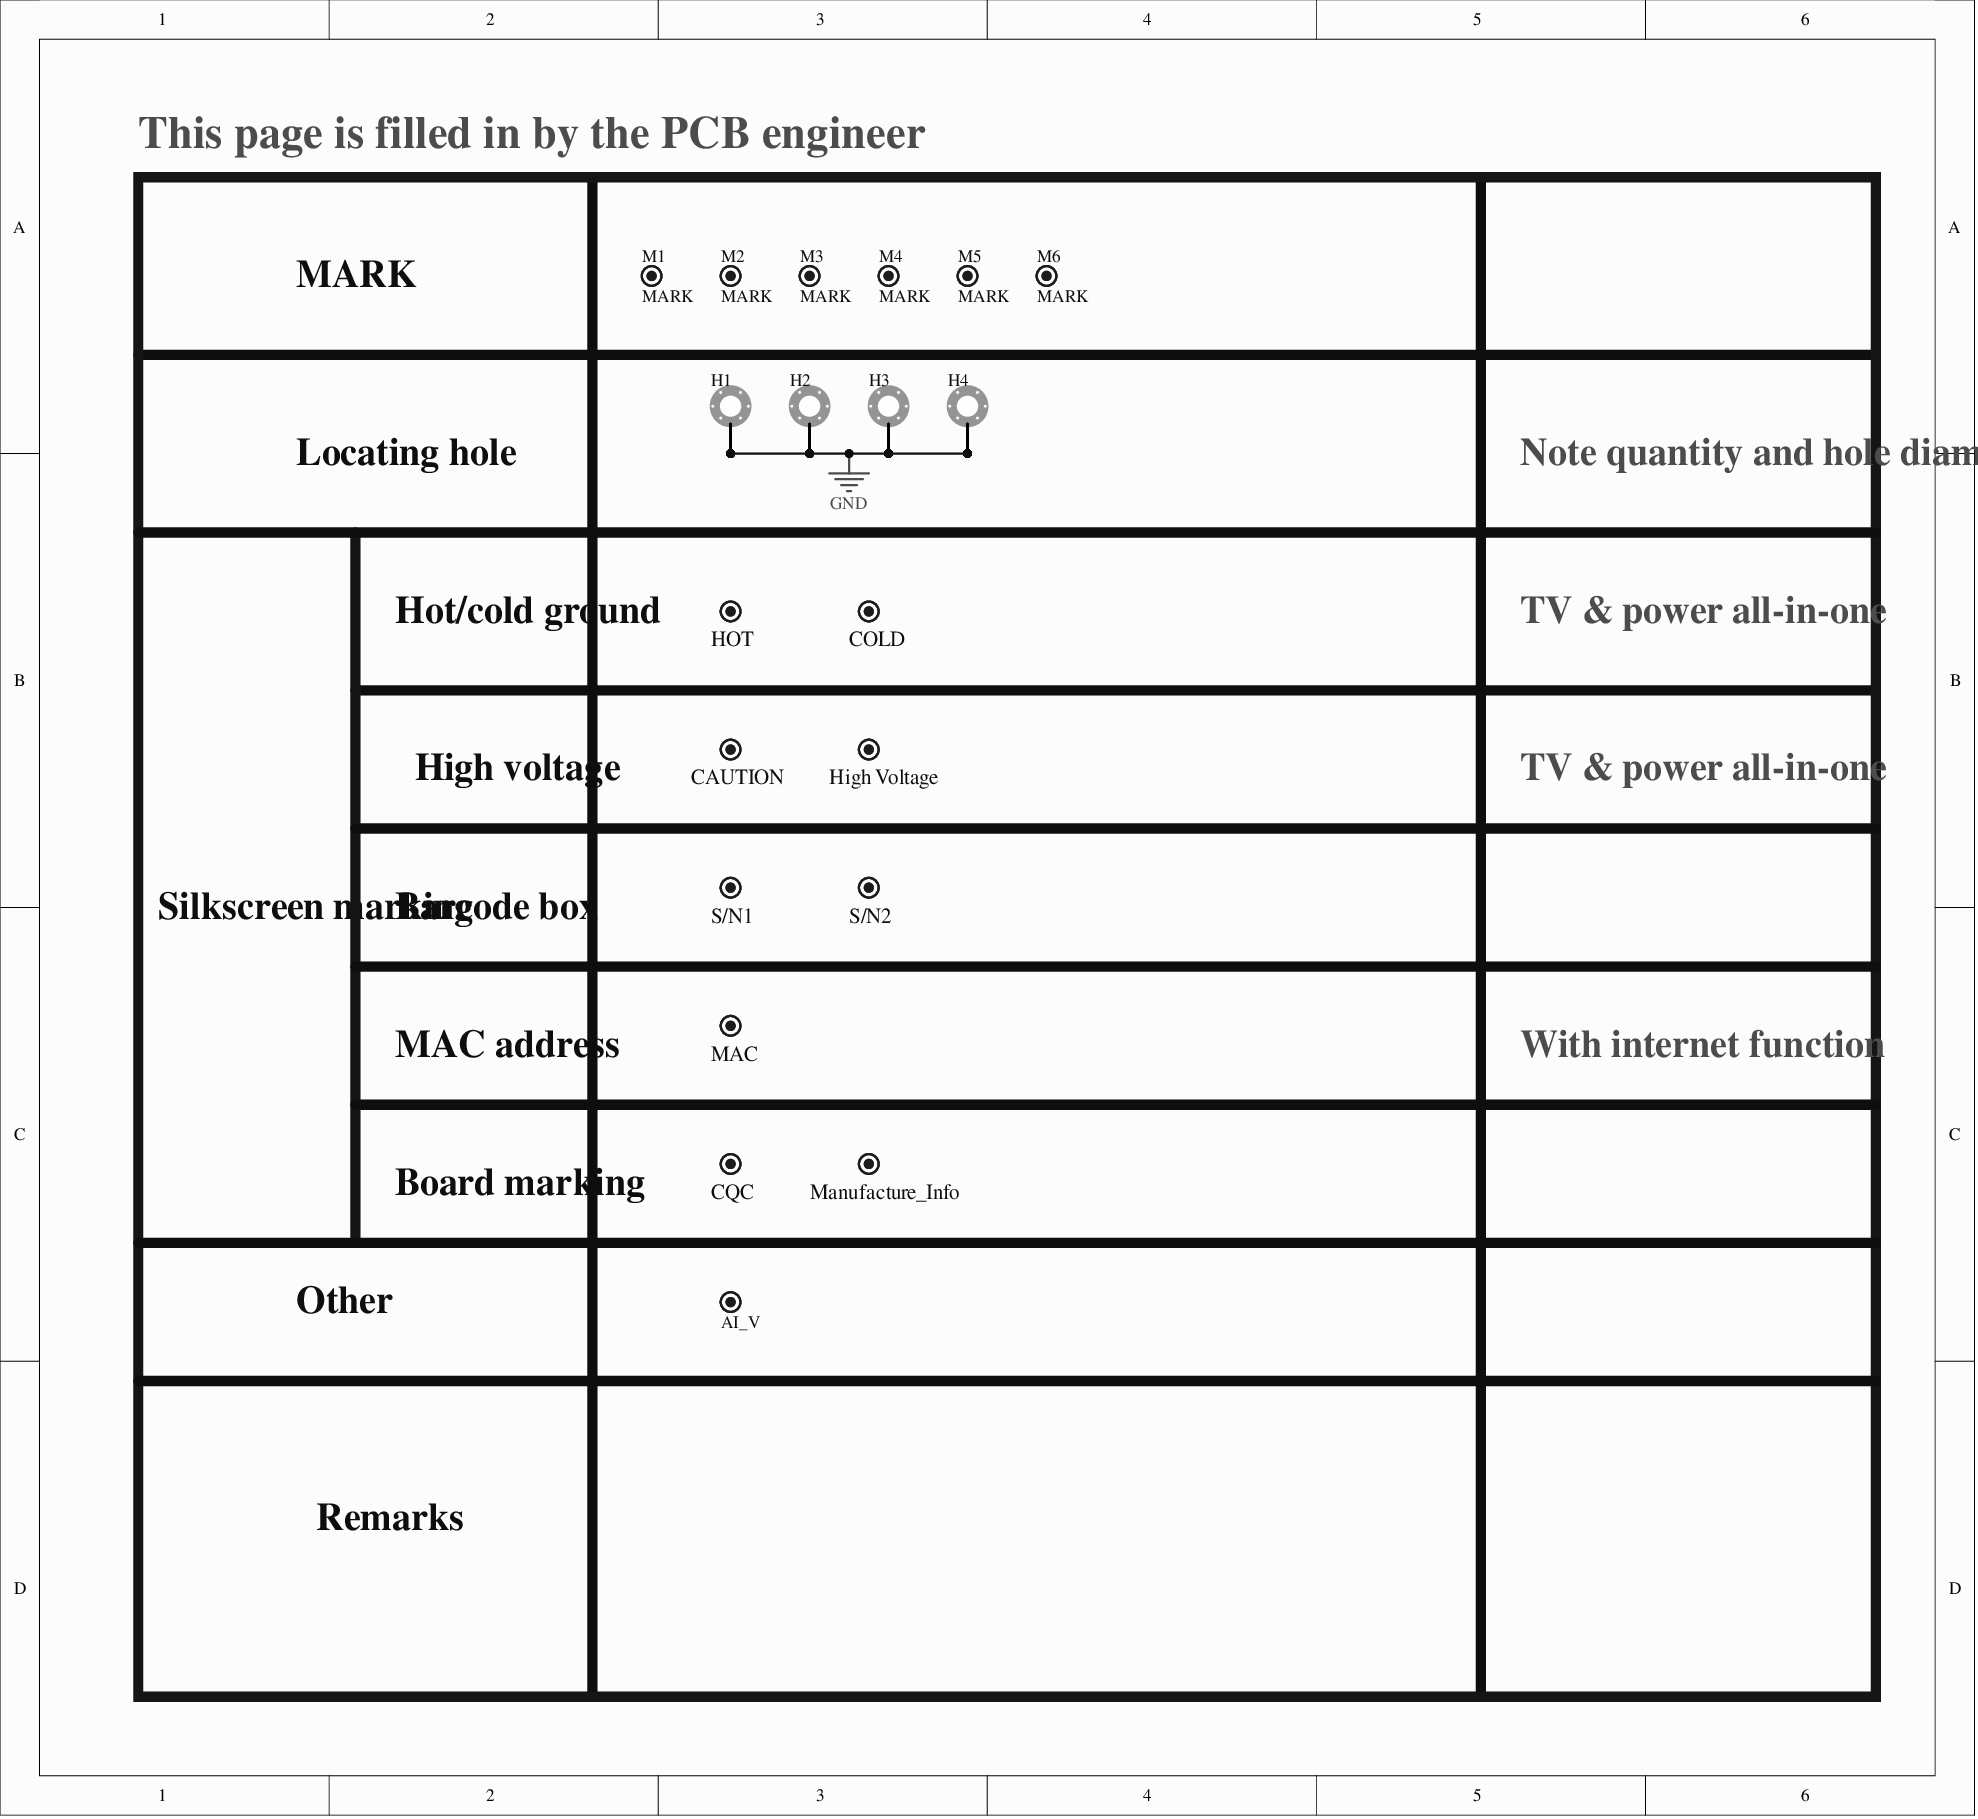
[diagram p0: MISC84395-3.SchDoc]
# Altium project MISC84395-37.PrjPCB (part 1 of 13)
17 sheets, 951 parts. Net scope: global (net labels, ports and power ports of the same name join across sheets).
Board file: MISC84395.PcbDoc
Sheets:
  MISC84395-3.SchDoc
  MISC84395-5.SchDoc
  MISC84395-2.schdoc
  MISC84395-7.SchDoc
  MISC84395-8.SchDoc
  MISC84395-9.SchDoc
  MISC84395-10.SchDoc
  MISC84395-11.SchDoc
  MISC84395-12.SchDoc
  MISC84395-13.SchDoc
  MISC84395-14.SchDoc
  MISC84395-15.SchDoc
  MISC84395-16.SchDoc
  MISC84395-17.SchDoc
  MISC84395-18.SchDoc
  MISC84395-4.SchDoc
  MISC84395-19.SchDoc

## Sheet MISC84395-3.SchDoc
size 254 x 233 mm

### Parts
AI_V  AI_GRIPPER_V  [AI_GRIPPER_V]  (value not drawn)
CAUTION  CAUTION  [CAUTION]
COLD  COLD  [COLD]
CQC  CQC  [CQC]
H1  Location hole  [ASSE4.0C-3]  (value not drawn)
H2  Location hole  [ASSE4.0C-3]  (value not drawn)
H3  Location hole  [ASSE4.0C-3]  (value not drawn)
H4  Location hole  [ASSE4.0C-3]  (value not drawn)
High_Voltage  High Voltage  [High Voltage]
HOT  HOT  [HOT]
M1  MARK  [MARK]
M2  MARK  [MARK]
M3  MARK  [MARK]
M4  MARK  [MARK]
M5  MARK  [MARK]
M6  MARK  [MARK]
MAC  MAC  [Barcode]  (value not drawn)
Manufacture_Info  Manufacture_Info  [Manufacture_Info]
S/N1  Barcode  [Barcode]  (value not drawn)
S/N2  Barcode  [Barcode]  (value not drawn)

### Nets
GND: H1.1 H1.2 H1.3 H1.4 H1.5 H1.6 H2.1 H2.2 H2.3 H2.4 H2.5 H2.6 H3.1 H3.2 H3.3 H3.4 H3.5 H3.6 H4.1 H4.2 H4.3 H4.4 H4.5 H4.6

### Notes on the sheet
- This page is filled in by the PCB engineer
- MARK
- Locating hole
- Note quantity and hole diameter
- (near HOT) Hot/cold ground
- TV & power all-in-one
- High voltage
- Silkscreen marking
- Barcode box
- MAC address
- With internet function
- Board marking
- Other
- Remarks

### Library data of the parts
H1-H4 = Location hole-D
M1-M6 = MARK-D
MAC = Barcode

## Sheet MISC84395-5.SchDoc
size 254 x 322 mm
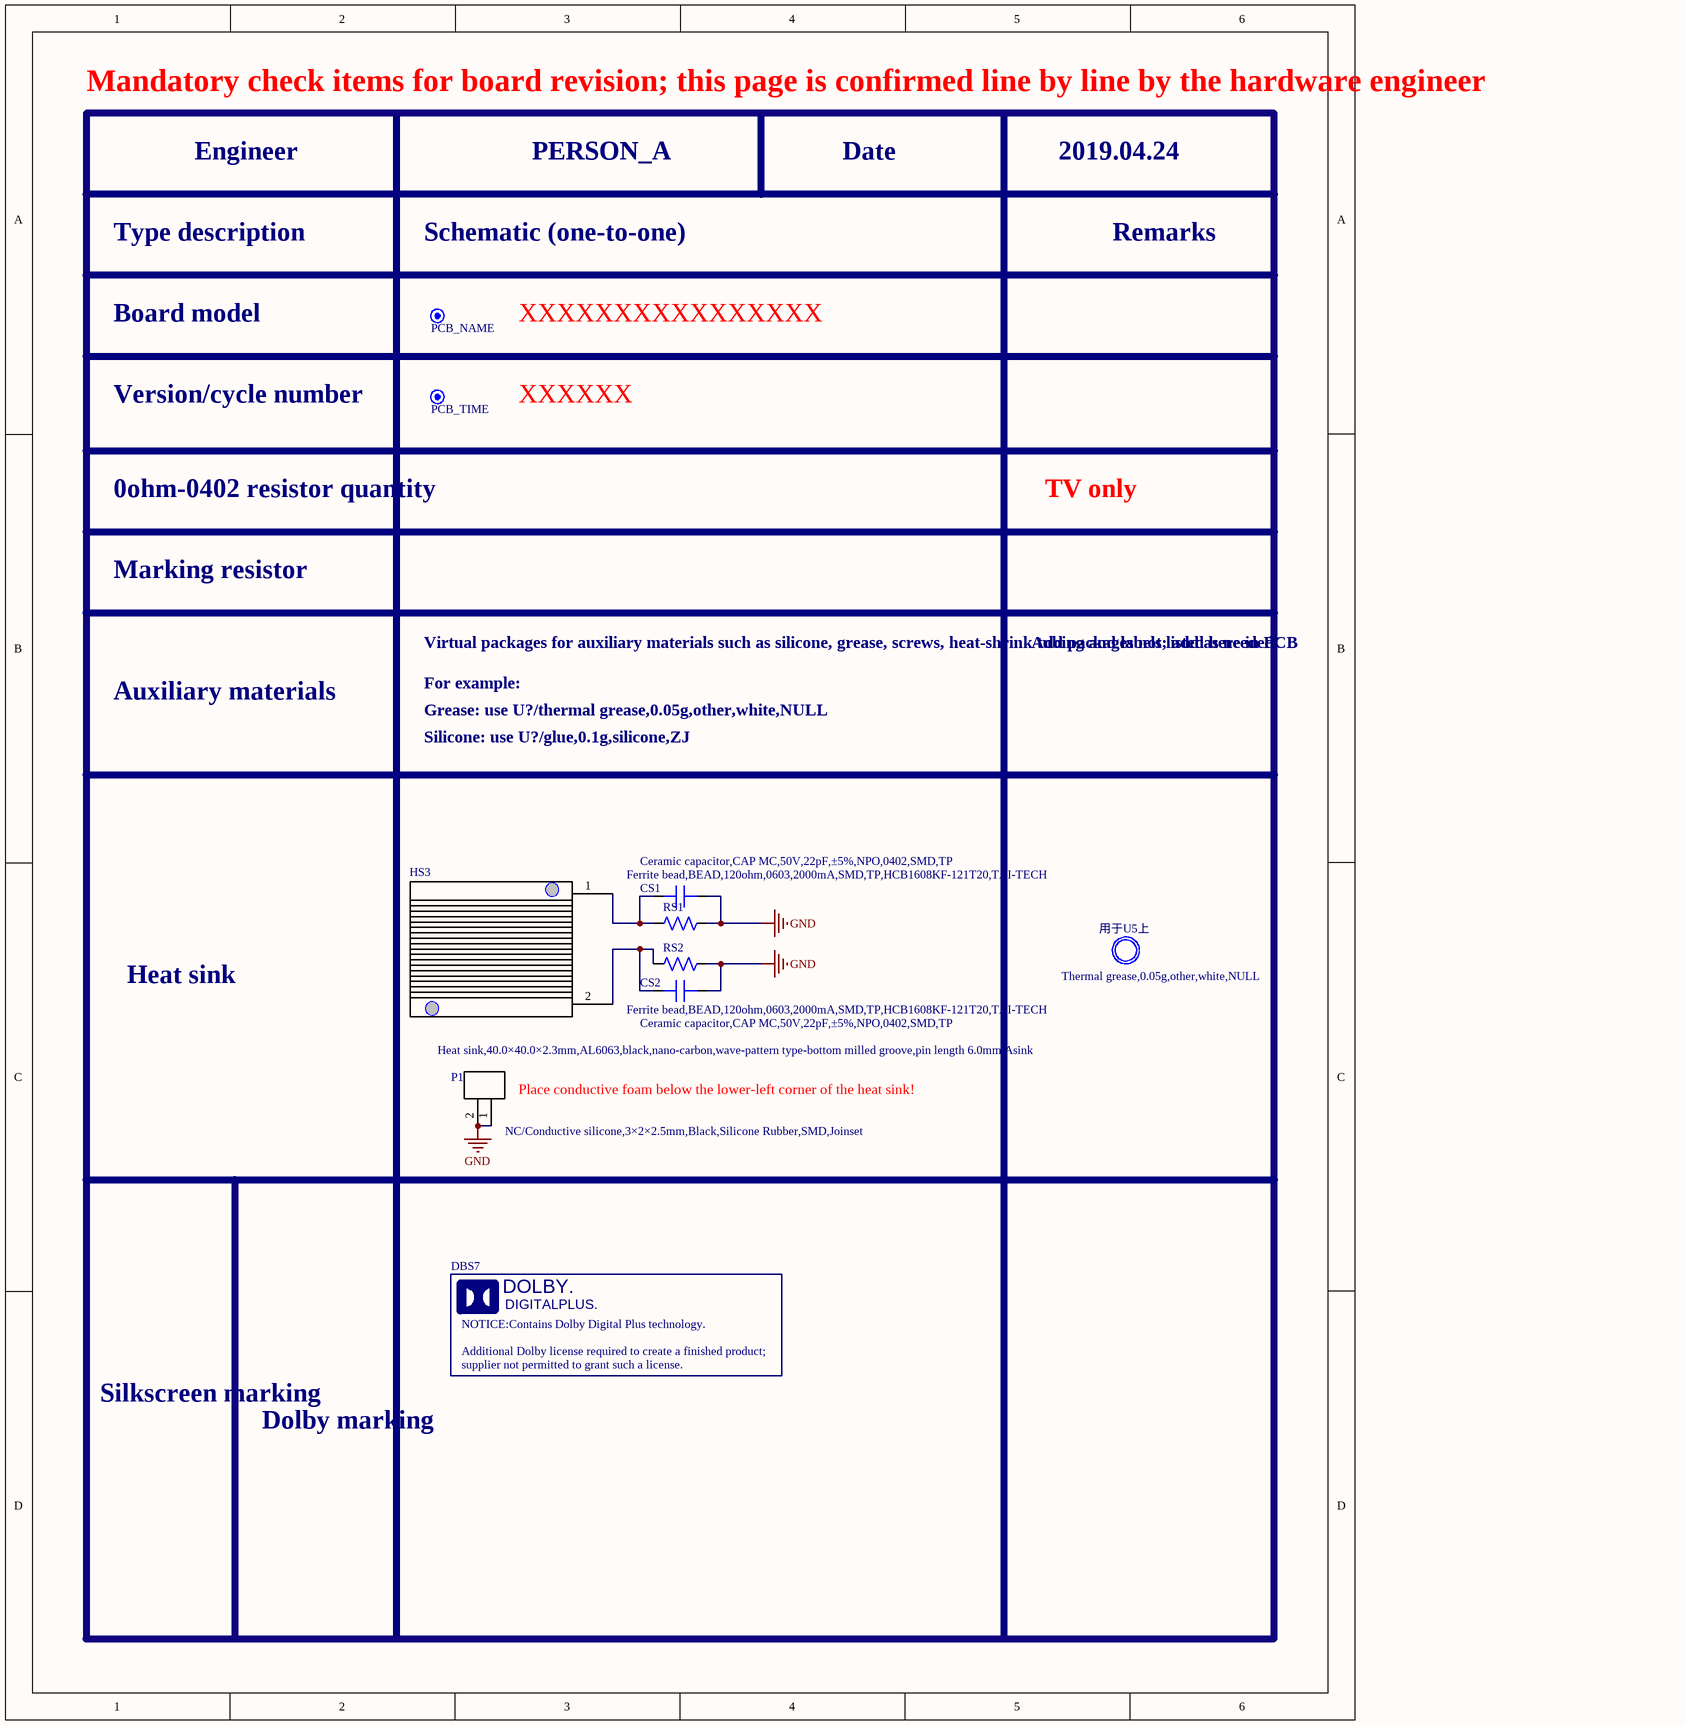
[diagram p1: MISC84395-5.SchDoc]

### Parts
CS1  Ceramic capacitor,CAP MC,50V,22pF,±5%,NPO,0402,SMD,TP  [C0402]
CS2  Ceramic capacitor,CAP MC,50V,22pF,±5%,NPO,0402,SMD,TP  [C0402]
DBS7  DOLBY PLUS  [DOLBY PLUS-SILK]  (value not drawn)
HS3  Heat sink,40.0×40.0×2.3mm,AL6063,black,nano-carbon,wave-pattern type-bottom milled groove,pin length 6.0mm,Asink  [HS(40*40*2.3)-1]
P1  NC/Conductive silicone,3×2×2.5mm,Black,Silicone Rubber,SMD,Joinset  [Silica gel(3*2*2.5)]
RS1  Ferrite bead,BEAD,120ohm,0603,2000mA,SMD,TP,HCB1608KF-121T20,TAI-TECH  [R0603]
RS2  Ferrite bead,BEAD,120ohm,0603,2000mA,SMD,TP,HCB1608KF-121T20,TAI-TECH  [R0603]
XXXXXX  PCB_TIME  [PCB_TIME]
XXXXXXXXXXXXXXXX  PCB_NAME  [PCB_NAME]
用于U5上  Thermal grease,0.05g,other,white,NULL  [Heat-Shrinkable Tube]

### Nets
GND: CS1.2 CS2.2 P1.1 P1.2 RS1.1 RS2.2
NetCS1_1: CS1.1 HS3.1 RS1.2
NetCS2_1: CS2.1 HS3.2 RS2.1

### Notes on the sheet
- Mandatory check items for board revision; this page is confirmed line by line by the hardware engineer
- Engineer
- PERSON_A
- Date
- 2019.04.24
- Type description
- Schematic (one-to-one)
- Remarks
- Board model
- Version/cycle number
- 0ohm-0402 resistor quantity
- TV only
- Marking resistor
- Virtual packages for auxiliary materials such as silicone, grease, screws, heat-shrink tubing and labels; add as needed
- Add packages not listed here in PCB
- Auxiliary materials
- For example:
- Grease: use U?/thermal grease,0.05g,other,white,NULL
- Silicone: use U?/glue,0.1g,silicone,ZJ
- Heat sink
- (near P1) Place conductive foam below the lower-left corner of the heat sink!
- Silkscreen marking
- Dolby marking

### Library data of the parts
CS1 CS2 = 1000pF-0402-X7R-±10%-50V-D
HS3 = 004.040.0002110-DLMI: Heat sink,AL6063,40.0×40.0×2.3mm,black,nano-carbon,wave-pattern type-bottom milled groove,Asink-DLMI
P1 = 导电硅胶,3×2×2.5mm,Black,Silicone Rubber,SMD,Joinset: EVA
RS1 RS2 = 0ohm-0603-±5%-1/10W-D
用于U5上 = Φ12mm×12mm-黑色-125度(UL认证)-D